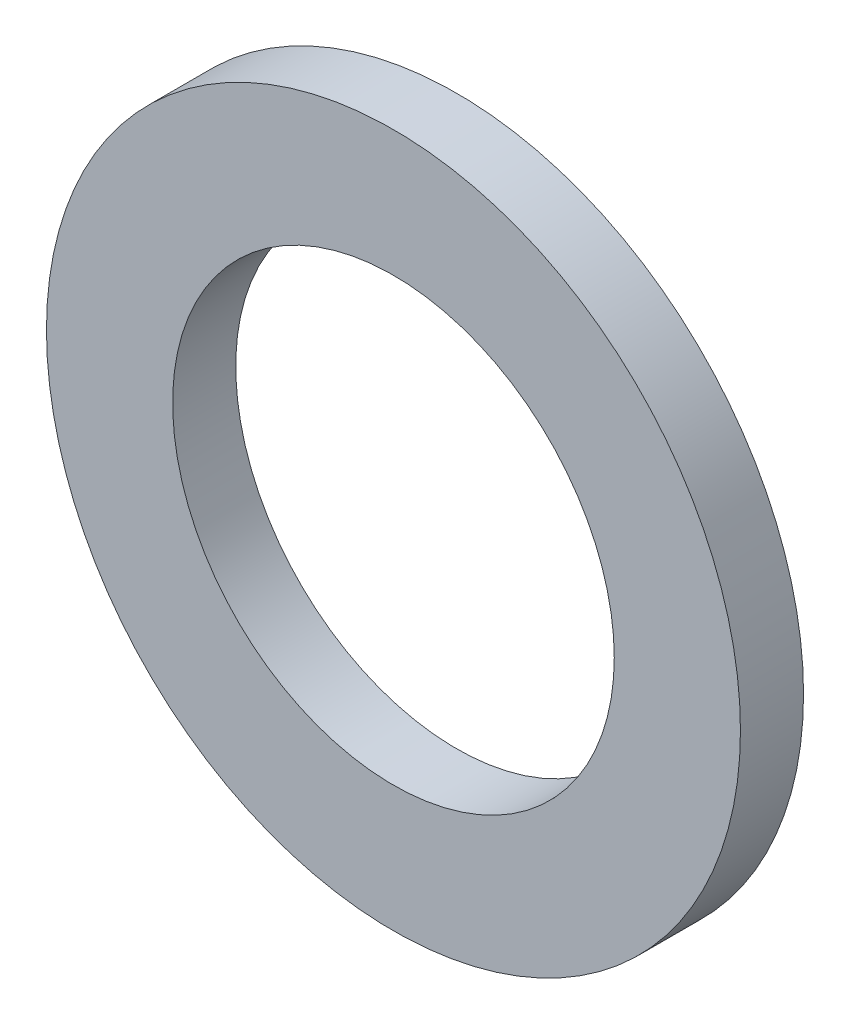
from build123d import *

# Parameters (mm, degrees)
SKETCH1_R           = 11
SKETCH1_R_2         = 7
BOSS_EXTRUDE1_DEPTH = 2


with BuildPart() as part:
    # Sketch1 → Boss-Extrude1 (new body)
    with BuildSketch(Plane.XY):
        Circle(SKETCH1_R)
        Circle(SKETCH1_R_2, mode=Mode.SUBTRACT)
    extrude(amount=BOSS_EXTRUDE1_DEPTH)


solid = part.part
